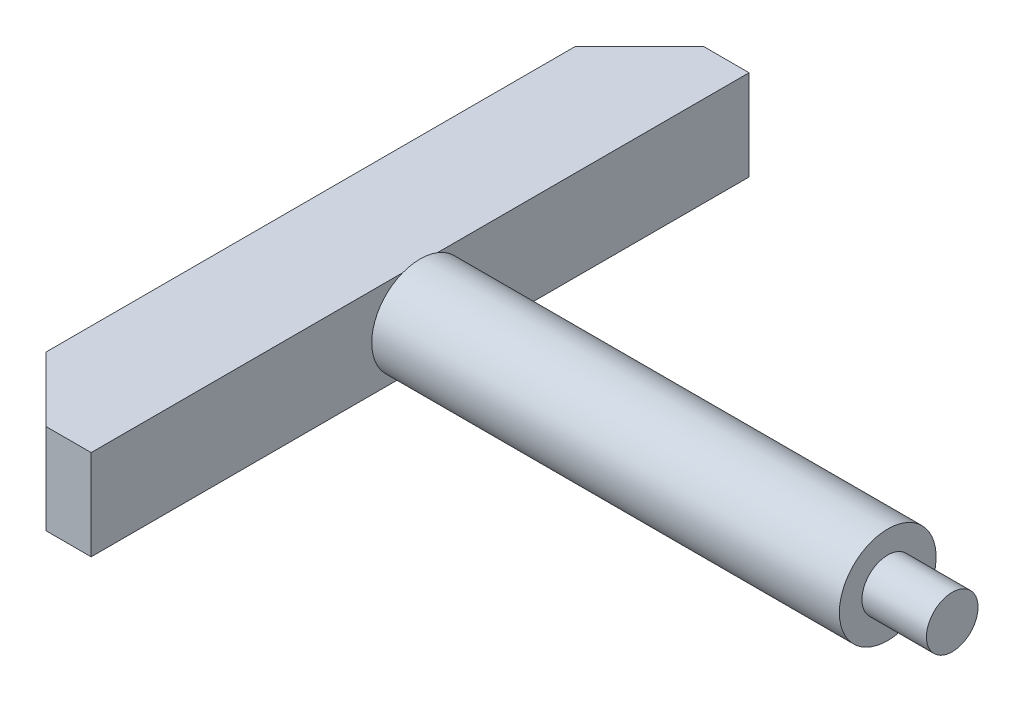
from build123d import *

# Parameters (mm, degrees)
SKETCH2_W           = 204
SKETCH2_H           = 28
BOSS_EXTRUDE1_DEPTH = 34
CHAMFER1_SIZE       = 20


with BuildPart() as part:
    # Sketch1 → Revolve1 (revolve)
    with BuildSketch(Plane.XY, mode=Mode.PRIVATE) as revolve1_sk:
        Polygon((0, 0), (0, 15), (145, 15), (145, 8), (165, 8), (165, 0), align=None)
    revolve(revolve1_sk.sketch.rotate(Axis((0, 0, 0), (1, 0, 0)), 90), axis=Axis((0, 0, 0), (1, 0, 0)))

    # Sketch2 → Boss-Extrude1 (add)
    with BuildSketch(Plane.ZY):
        Rectangle(SKETCH2_W, SKETCH2_H)
    extrude(amount=BOSS_EXTRUDE1_DEPTH)

    # Chamfer1
    chamfer1_edges = [part.edges().sort_by_distance(p)[0] for p in [
        (-34, 0, -102),
        (-34, 0, 102),
    ]]
    chamfer(chamfer1_edges, length=CHAMFER1_SIZE)


solid = part.part
